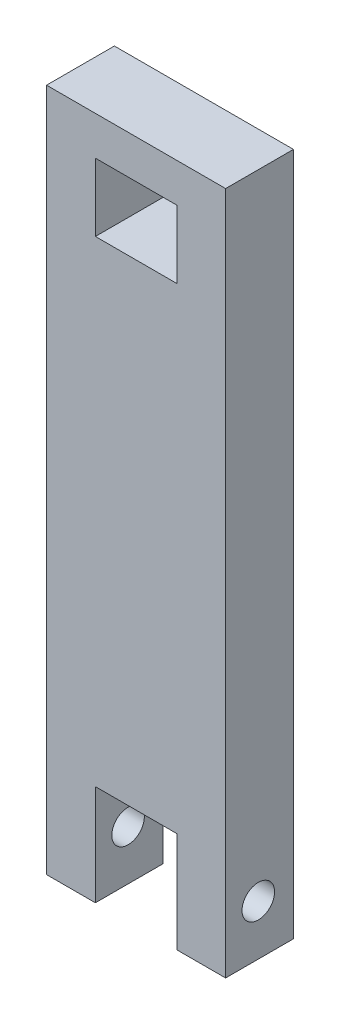
SolidWorks part; units mm, degrees
material "1060 合金"
ref_plane "前视基准面" through (0, 0, 0) normal (0, 0, 1) x (1, 0, 0)
ref_plane "上视基准面" through (0, 0, 0) normal (0, 1, 0) x (1, 0, 0)
ref_plane "右视基准面" through (0, 0, 0) normal (1, 0, 0) x (0, 0, -1)
sketch "草图1" plane through (0, 0, 0) normal (0, 0, 1) x (1, 0, 0)
  line L1 (-33, -150) -> (-15, -150)
  line L2 (-33, -150) -> (-33, 90)
  line L3 (-33, 90) -> (-15, 90)
  line L4 (33, -150) -> (33, 90)
  line L5 (15, 90) -> (33, 90)
  line L6 (-33, -30) -> (134.7368, -30) construction
  line L7 (0, -112.9042) -> (-15, -112.9042)
  line L11 (-15, -112.9042) -> (-15, -150)
  line L12 (0, -112.9042) -> (15, -112.9042)
  line L13 (15, -112.9042) -> (15, -150)
  line L14 (15, -150) -> (33, -150)
  line L15 (-15, 90) -> (15, 90)
  line L17 (0, 90) -> (0, 0) construction
  point P0 (0, 0)
  point P20 (-0.265, 29.4071)
  dimension "D1" = 33
  dimension "D2" = 240
  dimension "D3" = 33
  dimension "D4" = 30
extrude "凸台-拉伸1" add sketch "草图1" along normal mid plane 25
hole_wizard "M14 螺纹孔1" positions "3D草图3" profile "草图4" tap size "M14" standard "GB"
sketch3d "3D草图3"
  line L1 (33, -150, 12.5) -> (33, -150, -12.5) construction
  point P0 (33, -131.5, 0.4516)
  dimension "D1" = 18.5
sketch "草图4" plane through (33, -131.5, 0.4516) normal (0, 1, 0) x (0, 0, -1)
  line L0 (0, 0) -> (0, 18)
  line L1 (0, 18) -> (6, 18)
  line L2 (6, 18) -> (6, 0)
  line L5 (6, 0) -> (0, 0)
  line L11 (0, -6.35) -> (0, 107.95) construction
  dimension "通孔螺纹孔钻头直径" = 12
  dimension "通孔螺纹孔钻头深度" = 18
mirror "镜向1" about plane through (0, 0, 0) normal (1, 0, 0) of "M14 螺纹孔1"
sketch "草图7" plane through (0, 90, 0) normal (0, 1, 0) x (1, 0, 0)
  line L4 (33, 12.5) -> (-33, 12.5)
  line L5 (-33, 12.5) -> (-33, -12.5)
  line L12 (-33, 12.5) -> (-33, -12.5)
  line L14 (-33, -12.5) -> (33, -12.5)
  line L15 (-33, -12.5) -> (33, -12.5)
  line L16 (33, 12.5) -> (-33, 12.5)
  line L18 (33, -12.5) -> (33, 12.5)
  line L19 (33, -12.5) -> (33, 12.5)
  dimension "D1" = 0
extrude "凸台-拉伸2" add sketch "草图7" along normal blind 12
sketch "草图8" plane through (0, 0, -12.5) normal (0, 0, -1) x (-1, 0, 0)
  line L0 (-33, 102) -> (-33, 104.2849)
  line L1 (-33, 104.2849) -> (-43.9081, 104.2849)
  line L2 (-43.9081, 104.2849) -> (-43.9081, 119.3738)
sketch "草图12" plane through (0, 0, -12.5) normal (0, 0, -1) x (-1, 0, 0)
  line L0 (-15, 87.7045) -> (26.7871, 87.7045) construction
  line L1 (-15, 62.7045) -> (15, 62.7045)
  line L2 (-15, 62.7045) -> (-15, 87.7045)
  line L3 (-15, 87.7045) -> (15, 87.7045)
  line L4 (15, 62.7045) -> (15, 87.7045)
  dimension "D1" = 25
  dimension "D2" = 25
sketch "草图14" plane through (0, 0, -12.5) normal (0, 0, -1) x (-1, 0, 0)
  line L0 (-15, 62.7045) -> (-15, 87.7045) construction
  line L1 (-15, 71.5645) -> (15, 71.5645)
  line L2 (-15, 71.5645) -> (-15, 96.5645)
  line L3 (-15, 96.5645) -> (15, 96.5645)
  line L4 (15, 71.5645) -> (15, 96.5645)
  line L5 (-15, 62.7045) -> (15, 62.7045) construction
  dimension "D1" = 25
  dimension "D2" = 30
  dimension "D3" = 8.86
extrude "切除-拉伸5" cut sketch "草图12" against normal through all both
